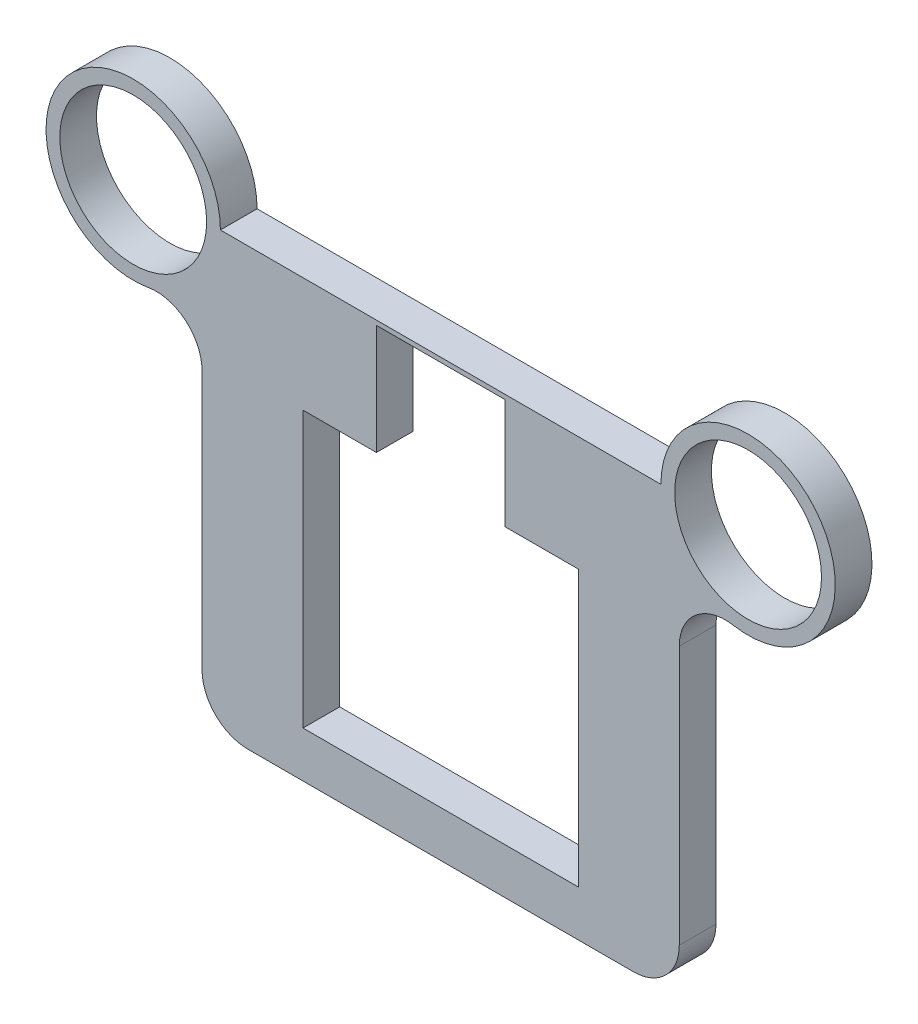
SolidWorks part; units mm, degrees
ref_plane "前视基准面" through (0, 0, 0) normal (0, 0, 1) x (1, 0, 0)
ref_plane "上视基准面" through (0, 0, 0) normal (0, 1, 0) x (1, 0, 0)
ref_plane "右视基准面" through (0, 0, 0) normal (1, 0, 0) x (0, 0, -1)
other "Configuration Table"
sketch "草图1" plane through (0, 0, 0) normal (0, 0, 1) x (1, 0, 0)
  line L0 (0, 57.5858) -> (0, -73.9808) construction
  line L1 (-107.643, 0) -> (127.2664, 0) construction
  line L2 (48.3923, 35.4467) -> (-47.6077, 35.4467)
  line L3 (-48.3923, 35.4467) -> (47.6077, 35.4467)
  line L4 (-52.3923, 6.881) -> (-52.3923, -49.5533)
  line L5 (-42.3923, -59.5533) -> (41.6077, -59.5533)
  line L6 (51.6077, 6.881) -> (51.6077, -49.5533)
  line L7 (-28.3637, -49.5533) -> (19.5228, -49.5533)
  line L8 (-30.3923, -49.5533) -> (-30.3923, 10.4467)
  line L9 (-30.3923, 10.4467) -> (29.6077, 10.4467)
  line L10 (29.6077, 10.4467) -> (29.6077, -49.5533)
  line L11 (29.6077, -49.5533) -> (19.5228, -49.5533)
  line L12 (-30.3923, -49.5533) -> (-28.3637, -49.5533)
  line L13 (-14.3923, 10.4467) -> (-14.3923, 34.4467)
  line L14 (-14.3923, 34.4467) -> (13.6077, 34.4467)
  line L15 (13.6077, 34.4467) -> (13.6077, 10.4467)
  arc A0 (-48.3923, 35.4467) -> (-64.1165, 16.7313) centre (-67.3923, 35.4467) ccw
  arc A1 (63.3318, 16.7313) -> (47.6077, 35.4467) centre (66.6077, 35.4467) ccw
  arc A2 (-52.3923, 6.881) -> (-64.1165, 16.7313) centre (-62.3923, 6.881) ccw
  arc A3 (63.3318, 16.7313) -> (51.6077, 6.881) centre (61.6077, 6.881) ccw
  circle A4 centre (-67.3923, 35.4467) radius 16
  circle A5 centre (66.6077, 35.4467) radius 16
  arc A6 (51.6077, -49.5533) -> (41.6077, -59.5533) centre (41.6077, -49.5533) cw
  arc A7 (-52.3923, -49.5533) -> (-42.3923, -59.5533) centre (-42.3923, -49.5533) ccw
  dimension "D1" = 38
  dimension "D2" = 38
  dimension "D5" = 20
  dimension "D6" = 20
  dimension "D9" = 32
  dimension "D10" = 32
  dimension "D11" = 10
  dimension "D7" = 62.3923
  dimension "D12" = 85
  dimension "D13" = 60
  dimension "D14" = 24
  dimension "D15" = 60
  dimension "D16" = 28
extrude "凸台-拉伸1" add sketch "草图1" along normal blind 8
